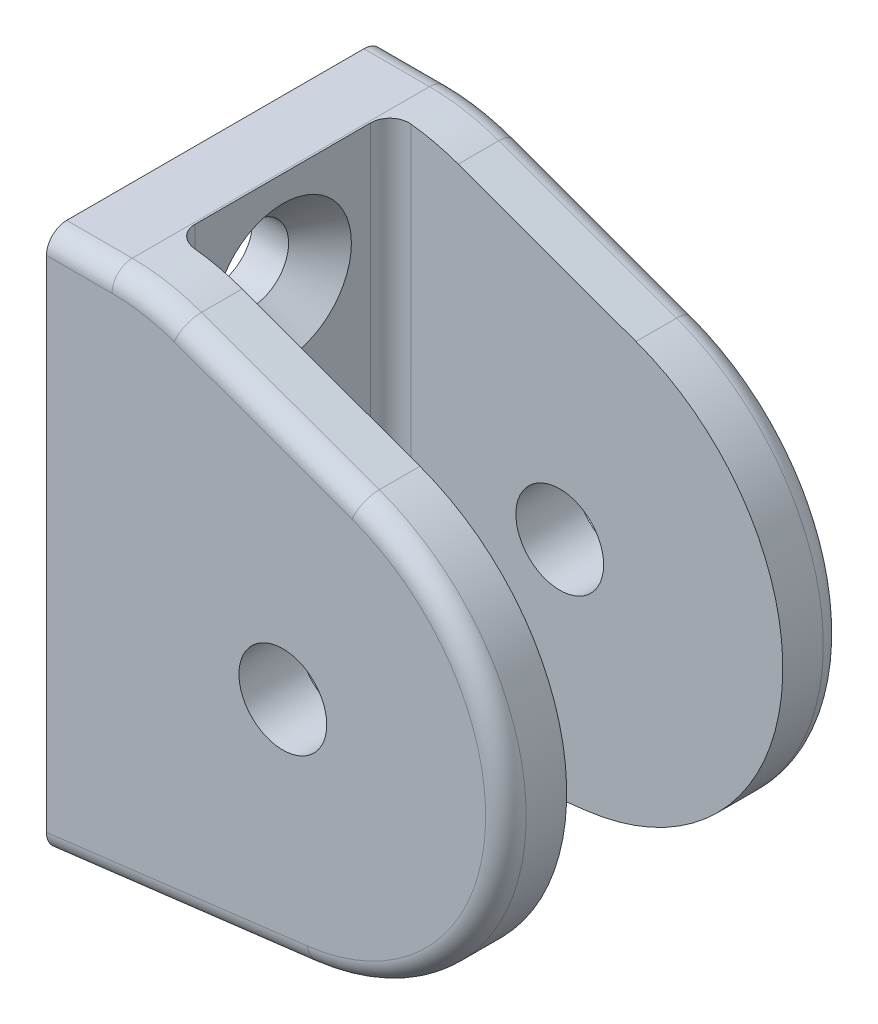
SolidWorks part; units mm, degrees
material "Q235-A"
ref_plane "前视基准面" through (0, 0, 0) normal (0, 0, 1) x (1, 0, 0)
ref_plane "上视基准面" through (0, 0, 0) normal (0, 1, 0) x (1, 0, 0)
ref_plane "右视基准面" through (0, 0, 0) normal (1, 0, 0) x (0, 0, -1)
sketch "草图2" plane through (0, 0, 0) normal (0, 0, 1) x (1, 0, 0)
  line L0 (0, 0) -> (0, 80)
  line L1 (0, 80) -> (9.7102, 80)
  line L3 (19.9708, 78.1908) -> (46.2961, 68.6091)
  line L4 (39.0251, 4.7917) -> (0, 0)
  arc A2 (46.2961, 68.6091) -> (39.0251, 4.7917) centre (35, 37.5732) cw
  arc A3 (9.7102, 80) -> (19.9708, 78.1908) centre (9.7102, 50) cw
  point P13 (15, 80)
  dimension "D1" = 80
  dimension "D6" = 30
  dimension "D2" = 15
  dimension "D3" = 20
  dimension "D4" = 83
  dimension "D5" = 35
extrude "凸台-拉伸1" add sketch "草图2" along normal mid plane 50
sketch "草图3" plane through (0, 0, 0) normal (0, 0, 1) x (1, 0, 0)
  line L0 (0, 80) -> (0, 0) construction
  line L1 (10, 90.1339) -> (78.113, 90.1339)
  line L2 (10, 90.1339) -> (10, -7.8866)
  line L3 (10, -7.8866) -> (78.113, -7.8866)
  line L4 (78.113, 90.1339) -> (78.113, -7.8866)
  dimension "D1" = 10
extrude "切除-拉伸1" cut sketch "草图3" against normal mid plane 32
sketch "草图4" plane through (0, 0, 25) normal (0, 0, 1) x (1, 0, 0)
  circle A0 centre (35, 37.5732) radius 6.5
  dimension "D1" = 13
extrude "切除-拉伸2" cut sketch "草图4" against normal through all
fillet "圆角1" radius 3 10 edges at (19.5125, 2.3958, -25) (67.8154, 33.8344, -25) (19.5125, 2.3958, 25) (67.8154, 33.8344, 25) (4.8551, 80, -25) (33.1335, 73.4, -25) (4.8551, 80, 25) (33.1335, 73.4, 25) (14.9196, 79.5442, -25) (14.9196, 79.5442, 25)
hole_wizard "打孔尺寸(%根据)内六角花形半沉头螺钉的类型1" positions "草图5" profile "草图6" countersink size "M10" standard "GB" end condition through all
sketch "草图5" plane through (10, 0, 0) normal (1, 0, 0) x (0, 0, -1)
  line L0 (-16, 79.9986) -> (16, 79.9986) construction
  line L1 (-22, 0) -> (22, 0) construction
  point P0 (0, 65.9986)
  point P2 (0, 15)
  dimension "D1" = 14
  dimension "D2" = 15
sketch "草图6" plane through (10, 65.9986, 0) normal (0, 1, 0) x (0, 0, -1)
  line L0 (0, 0) -> (0, 10)
  line L1 (0, 10) -> (5.5, 10)
  line L2 (5.5, 10) -> (5.5, 4.65)
  line L3 (5.5, 4.65) -> (10.15, 0)
  line L5 (10.15, 0) -> (0, 0)
  line L6 (-5.5, 4.65) -> (-10.15, 0) construction
  line L11 (0, -6.35) -> (0, 107.95) construction
  dimension "通孔孔直径" = 11
  dimension "通孔孔深度" = 10
  dimension "近端锥形沉头孔直径" = 20.3
  dimension "近端锥形沉头孔角度" = 90
fillet "圆角2" radius 3 2 edges at (10, 40.6132, -16) (10, 40.6132, 16)
